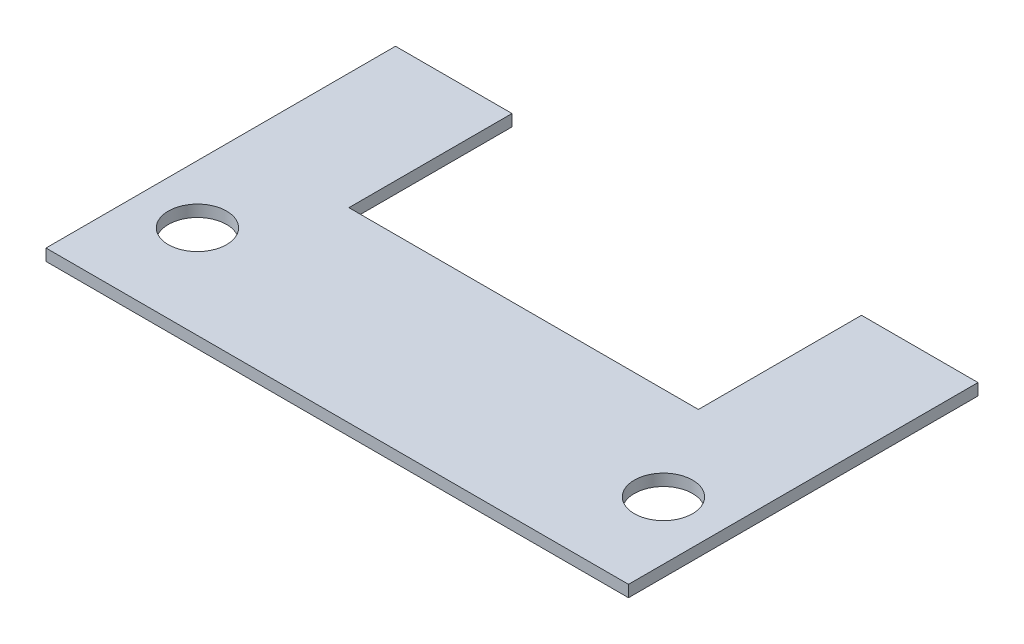
from build123d import *

# Parameters (mm, degrees)
SKETCH1_R           = 1.25
BOSS_EXTRUDE1_DEPTH = 0.5


with BuildPart() as part:
    # Sketch1 → Boss-Extrude1 (new body)
    with BuildSketch(Plane(origin=(0, 0, 0), x_dir=(1, 0, 0), z_dir=(0, 1, 0))):
        Polygon((-12.5, 0), (12.5, 0), (12.5, 15), (7.5, 15), (7.5, 8), (-7.5, 8), (-7.5, 15), (-12.5, 15), align=None)
        with Locations(Location((10, 4, 0), (0, 0, 270))):
            Circle(SKETCH1_R, mode=Mode.SUBTRACT)
        with Locations(Location((-10, 4, 0), (0, 0, 270))):
            Circle(SKETCH1_R, mode=Mode.SUBTRACT)
    extrude(amount=BOSS_EXTRUDE1_DEPTH)


solid = part.part
